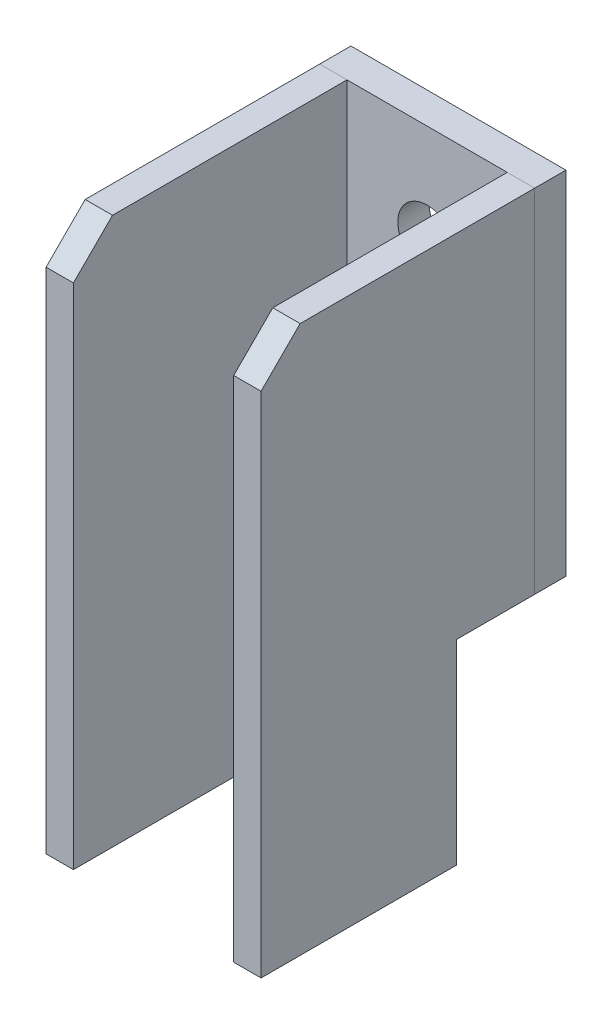
SolidWorks part; units mm, degrees
ref_plane "前视基准面" through (0, 0, 0) normal (0, 0, 1) x (1, 0, 0)
ref_plane "上视基准面" through (0, 0, 0) normal (0, 1, 0) x (1, 0, 0)
ref_plane "右视基准面" through (0, 0, 0) normal (1, 0, 0) x (0, 0, -1)
other "Configuration Table"
sketch "草图1" plane through (0, 0, 0) normal (0, 0, 1) x (1, 0, 0)
  line L1 (-55, -50) -> (55, -50)
  line L2 (-55, -50) -> (-55, 50)
  line L3 (-55, 50) -> (55, 50)
  line L4 (55, -50) -> (55, 50)
  line L5 (0, 50) -> (0, -50) construction
  line L6 (-55, 0) -> (55, 0) construction
  point P0 (0, 0)
  dimension "D1" = 110
  dimension "D2" = 100
extrude "凸台-拉伸1" add sketch "草图1" along normal blind 16
sketch "草图2" plane through (-55, 0, 0) normal (-1, 0, 0) x (0, 0, 1)
  line L9 (16, 50) -> (16, -130)
  line L12 (16, 50) -> (156, 50)
  line L13 (156, 50) -> (156, -230)
  line L14 (156, -230) -> (56, -230)
  line L15 (56, -230) -> (56, -130)
  line L16 (56, -130) -> (16, -130)
  dimension "D1" = 40
  dimension "D2" = 180
  dimension "D3" = 280
  dimension "D4" = 100
extrude "凸台-拉伸2" add sketch "草图2" against normal blind 14 separate body
chamfer "倒角1" distance 20 angle 45 1 edges at (-48, 50, 156)
mirror "镜向1" about plane through (0, 0, 0) normal (1, 0, 0) of bodies 107
sketch "草图3" plane through (0, 0, 0) normal (0, 0, -1) x (-1, 0, 0)
  circle A0 centre (0, 0) radius 15
  dimension "D1" = 30
extrude "切除-拉伸1" cut sketch "草图3" against normal up to next (16 mm away)
sketch "草图4" plane through (0, -50, 0) normal (0, -1, 0) x (1, 0, 0)
  line L1 (-55, 16) -> (55, 16)
  line L2 (-55, 16) -> (-55, 0)
  line L3 (-55, 0) -> (55, 0)
  line L4 (55, 16) -> (55, 0)
  line L5 (-55, 16) -> (-55, 56) construction
  dimension "D1" = 16
extrude "凸台-拉伸3" add sketch "草图4" along normal up to vertex (80 mm away) up to point (-55, -130, 16)
